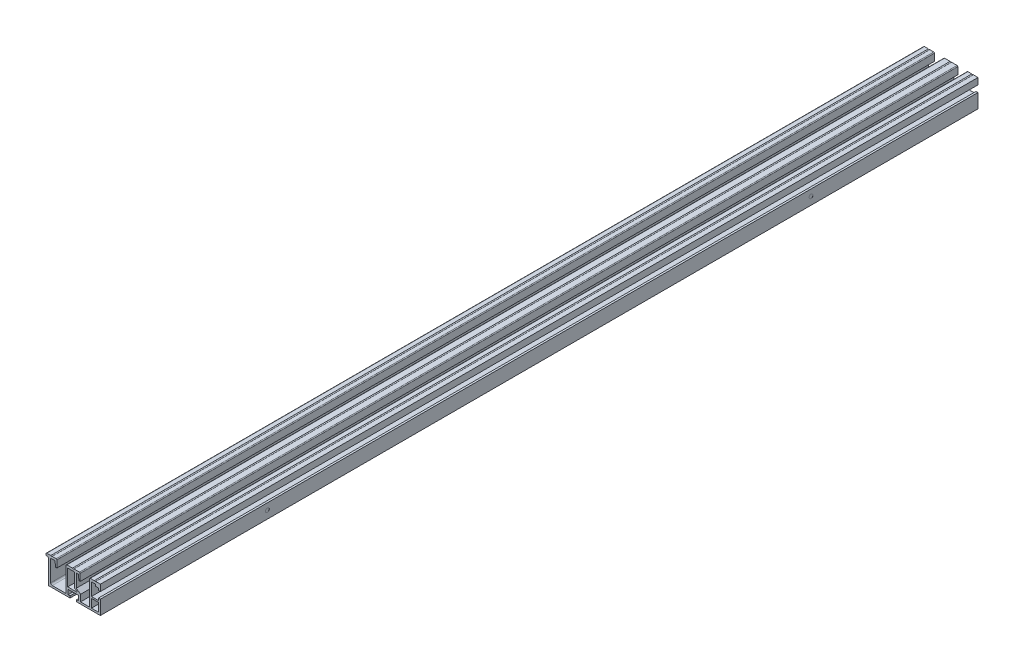
from build123d import *

# Parameters (mm, degrees)
SKETCH_1_W               = 9
SKETCH_1_H               = 11
EXTRUDE_1_DEPTH          = 565
CUT_EXTRUDE_1_DEPTH      = 571.246657158
CUT_EXTRUDE_1_DEPTH_BACK = 571.246657158
SKETCH_3_R               = 2.5
CUT_EXTRUDE_2_DEPTH      = 0.1


with BuildPart() as part:
    # 草图1 → 凸台-拉伸1 (new, symmetric)
    with BuildSketch(Plane.XY):
        with BuildLine():
            Line((-28.5, 32), (-27.5, 25))
            Line((-27.5, 25), (-26, 25))
            Line((-26, 25), (-26, 34))
            ThreePointArc((-26, 34), (-26.292893219, 34.707106781), (-27, 35))
            Line((-27, 35), (-34.1, 35))
            ThreePointArc((-34.1, 35), (-35, 34.7), (-35.9, 35))
            Line((-35.9, 35), (-43, 35))
            ThreePointArc((-43, 35), (-43.707106781, 34.707106781), (-44, 34))
            Line((-44, 34), (-44, 2.5))
            Line((-44, 2.5), (-62, 2.5))
            ThreePointArc((-62, 2.5), (-63.414213562, 3.085786438), (-64, 4.5))
            Line((-64, 4.5), (-64, 31))
            ThreePointArc((-64, 31), (-63.707106781, 31.707106781), (-63, 32))
            Line((-63, 32), (-58.5, 32))
            Line((-58.5, 32), (-57.5, 25))
            Line((-57.5, 25), (-56, 25))
            Line((-56, 25), (-56, 34))
            ThreePointArc((-56, 34), (-56.292893219, 34.707106781), (-57, 35))
            Line((-57, 35), (-62.1, 35))
            ThreePointArc((-62.1, 35), (-63, 34.7), (-63.9, 35))
            Line((-63.9, 35), (-69, 35))
            ThreePointArc((-69, 35), (-69.707106781, 34.707106781), (-70, 34))
            Line((-70, 34), (-70, 32))
            Line((-70, 32), (-68, 32))
            ThreePointArc((-68, 32), (-67.292893219, 31.707106781), (-67, 31))
            Line((-67, 31), (-67, 0))
            Line((-67, 0), (-39, 0))
            Line((-39, 0), (-39, 2.5))
            Line((-39, 2.5), (-41.5, 2.5))
            Line((-41.5, 2.5), (-41.5, 8.5))
            Line((-41.5, 8.5), (-28.006, 8.5))
            Line((-28.006, 8.5), (-28.006, 2.5))
            Line((-28.006, 2.5), (-30.5, 2.5))
            Line((-30.5, 2.5), (-30.5, 0))
            Line((-30.5, 0), (0, 0))
            Line((0, 0), (0, 18.25))
            Line((0, 18.25), (-2.5, 18.25))
            Line((-2.5, 18.25), (-2.5, 15.5))
            Line((-2.5, 15.5), (-11.5, 15.5))
            Line((-11.5, 15.5), (-11.5, 31))
            ThreePointArc((-11.5, 31), (-11.207106781, 31.707106781), (-10.5, 32))
            Line((-10.5, 32), (-6.5, 32))
            Line((-6.5, 32), (-6.5, 29.5))
            Line((-6.5, 29.5), (-2.5, 29.5))
            Line((-2.5, 29.5), (-2.5, 26.75))
            Line((-2.5, 26.75), (0, 26.75))
            Line((0, 26.75), (0, 35))
            Line((0, 35), (-6.1, 35))
            ThreePointArc((-6.1, 35), (-7, 34.7), (-7.9, 35))
            Line((-7.9, 35), (-13, 35))
            ThreePointArc((-13, 35), (-13.707106781, 34.707106781), (-14, 34))
            Line((-14, 34), (-14, 2.5))
            Line((-14, 2.5), (-25.5, 2.5))
            Line((-25.5, 2.5), (-25.5, 11))
            Line((-25.5, 11), (-31, 15))
            Line((-31, 15), (-31, 32))
            Line((-31, 32), (-28.5, 32))
        make_face()
        with Locations((-7, 8)):
            Rectangle(SKETCH_1_W, SKETCH_1_H, mode=Mode.SUBTRACT)
        with BuildLine():
            Line((-42, 11), (-42, 32))
            Line((-42, 32), (-33, 32))
            Line((-33, 32), (-33, 13.981550817))
            Line((-33, 13.981550817), (-30.143873685, 11.904368042))
            ThreePointArc((-30.143873685, 11.904368042), (-29.962468198, 11.345377914), (-30.437959534, 11))
            Line((-30.437959534, 11), (-42, 11))
        make_face(mode=Mode.SUBTRACT)
    extrude(amount=EXTRUDE_1_DEPTH, both=True)

    # 草图2 → 切除-拉伸1 (cut, two sides: drawn at the far end of the back side and taken through both)
    with BuildSketch(Plane(origin=(0, 2.5, 0), x_dir=(1, 0, 0), z_dir=(0, 1, 0)).offset(-CUT_EXTRUDE_1_DEPTH_BACK)):
        with BuildLine():
            Line((-15.5, -205.5), (-15.5, -164.5))
            ThreePointArc((-15.5, -164.5), (-20, -160), (-24.5, -164.5))
            Line((-24.5, -164.5), (-24.5, -205.5))
            ThreePointArc((-24.5, -205.5), (-20, -210), (-15.5, -205.5))
        make_face()
        with BuildLine():
            Line((-45.5, 95.5), (-45.5, 54.5))
            ThreePointArc((-45.5, 54.5), (-50, 50), (-54.5, 54.5))
            Line((-54.5, 54.5), (-54.5, 95.5))
            ThreePointArc((-54.5, 95.5), (-50, 100), (-45.5, 95.5))
        make_face()
        with BuildLine():
            Line((-45.5, -95.5), (-45.5, -54.5))
            ThreePointArc((-45.5, -54.5), (-50, -50), (-54.5, -54.5))
            Line((-54.5, -54.5), (-54.5, -95.5))
            ThreePointArc((-54.5, -95.5), (-50, -100), (-45.5, -95.5))
        make_face()
        with BuildLine():
            Line((-15.5, 205.5), (-15.5, 164.5))
            ThreePointArc((-15.5, 164.5), (-20, 160), (-24.5, 164.5))
            Line((-24.5, 164.5), (-24.5, 205.5))
            ThreePointArc((-24.5, 205.5), (-20, 210), (-15.5, 205.5))
        make_face()
    extrude(amount=CUT_EXTRUDE_1_DEPTH + CUT_EXTRUDE_1_DEPTH_BACK, mode=Mode.SUBTRACT)

    # 草图3 → 切除-拉伸2 (cut)
    with BuildSketch(Plane(origin=(0, 0, 0), x_dir=(0, 0, -1), z_dir=(1, 0, 0))):
        with Locations((-350, 10)):
            Circle(SKETCH_3_R)
        with Locations(Location((350, 10, 0), (0, 0, 180))):
            Circle(SKETCH_3_R)
    extrude(amount=-CUT_EXTRUDE_2_DEPTH, mode=Mode.SUBTRACT)


solid = part.part
